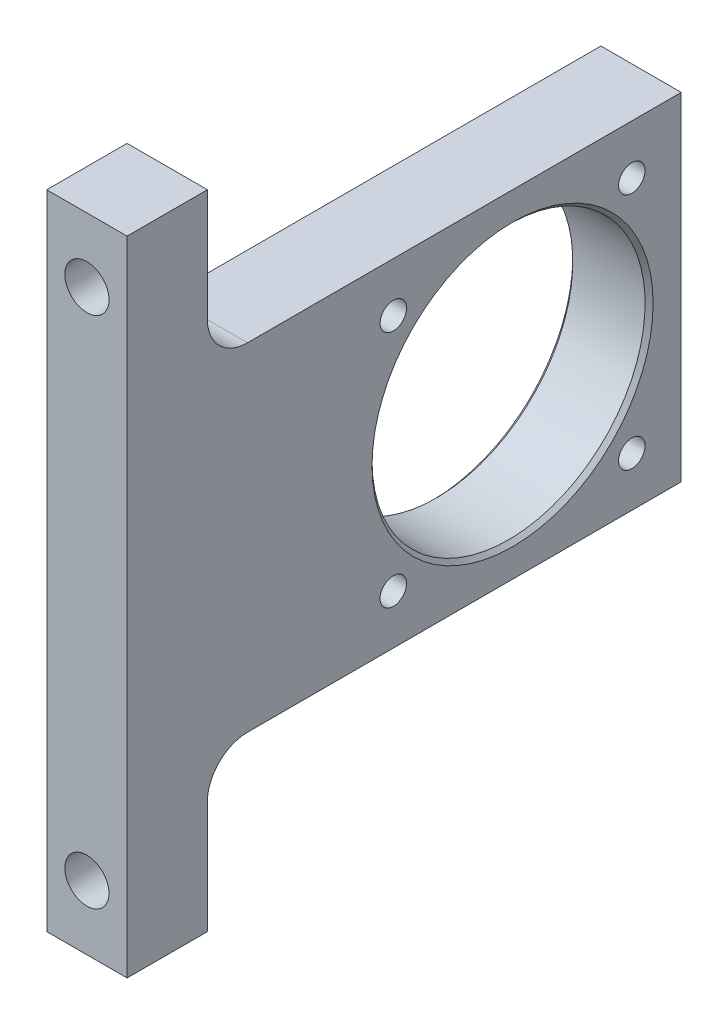
SolidWorks part; units mm, degrees
ref_plane "Front" through (0, 0, 0) normal (0, 0, 1) x (1, 0, 0)
ref_plane "Top" through (0, 0, 0) normal (0, 1, 0) x (1, 0, 0)
ref_plane "Right" through (0, 0, 0) normal (1, 0, 0) x (0, 0, -1)
sketch "Sketch1" plane through (0, 0, 0) normal (1, 0, 0) x (0, 0, -1)
  line L0 (0, -40) -> (0, 40)
  line L1 (0, 40) -> (10, 40)
  line L2 (10, 40) -> (10, 21)
  line L3 (10, 21) -> (69, 21)
  line L4 (69, 21) -> (69, -21)
  line L5 (69, -21) -> (10, -21)
  line L6 (10, -21) -> (10, -40)
  line L7 (10, -40) -> (0, -40)
  line L8 (0, 0) -> (69, 0) construction
  dimension "D1" = 69
  dimension "D2" = 10
  dimension "D3" = 42
  dimension "D4" = 80
extrude "Boss-Extrude1" add sketch "Sketch1" along normal blind 10
sketch "Sketch2" plane through (10, 0, 0) normal (1, 0, 0) x (0, 0, -1)
  line L0 (0, 40) -> (0, -40) construction
  circle A0 centre (48, 0) radius 17
  dimension "D2" = 34
  dimension "D1" = 48
extrude "Cut-Extrude1" cut sketch "Sketch2" against normal through all
hole_wizard "Ø5.5 (5.5) Diameter Hole1" positions "Sketch4" profile "Sketch3" hole size "Ø5.5" standard "ISO" end condition through all
sketch "Sketch4" plane through (0, 0, 0) normal (0, 0, 1) x (1, 0, 0)
  line L0 (0, 0) -> (10, 0) construction
  line L1 (0, 40) -> (0, -40) construction
  line L2 (10, 40) -> (10, -40) construction
  point P0 (5, 32)
  point P1 (5, -32)
  dimension "D1" = 64
  dimension "D2" = 5
sketch "Sketch3" plane through (5, 32, 0) normal (1, 0, 0) x (0, -1, 0)
  line L0 (0, 0) -> (0, 69)
  line L1 (0, 69) -> (2.75, 69)
  line L2 (2.75, 69) -> (2.75, 0)
  line L5 (2.75, 0) -> (0, 0)
  line L11 (0, -6.35) -> (0, 107.95) construction
  dimension "Thru Hole Dia." = 5.5
  dimension "Thru Hole Depth" = 69
hole_wizard "M4 Tapped Hole1" positions "Sketch6" profile "Sketch5" tap size "M4" standard "ISO" end condition through all
sketch "Sketch6" plane through (10, 0, 0) normal (1, 0, 0) x (0, 0, -1)
  line L2 (22.6804, 0) -> (73.7683, 0) construction
  line L5 (48, -25.0982) -> (48, 26.5068) construction
  line L7 (29.679, -18.321) -> (67.5069, 19.5069) construction
  line L9 (28.809, 19.191) -> (65.2215, -17.2215) construction
  circle A0 centre (48, 0) radius 21 construction
  point P0 (33.1508, 14.8492)
  point P1 (62.8492, 14.8492)
  point P3 (62.8492, -14.8492)
  point P5 (33.1508, -14.8492)
  dimension "D1" = 42
  dimension "D2" = 45
  dimension "D3" = 45
sketch "Sketch5" plane through (10, 14.8492, -33.1508) normal (0, 1, 0) x (0, 0, -1)
  line L0 (0, 0) -> (0, 10)
  line L1 (0, 10) -> (1.65, 10)
  line L2 (1.65, 10) -> (1.65, 0)
  line L5 (1.65, 0) -> (0, 0)
  line L11 (0, -6.35) -> (0, 107.95) construction
  dimension "Thru Tap Drill Dia." = 3.3
  dimension "Thru Tap Drill Depth" = 10
cosmetic thread "Hole Thread1" parameters "D2"=4
cosmetic thread "Hole Thread2" parameters "D2"=4
cosmetic thread "Hole Thread3" parameters "D2"=4
cosmetic thread "Hole Thread4" parameters "D2"=4
fillet "Fillet1" radius 5 2 edges at (5, 21, -10) (5, -21, -10)
chamfer "Chamfer1" distance 0.5 angle 45 2 edges at (0, 0, -65) (10, 0, -65)
